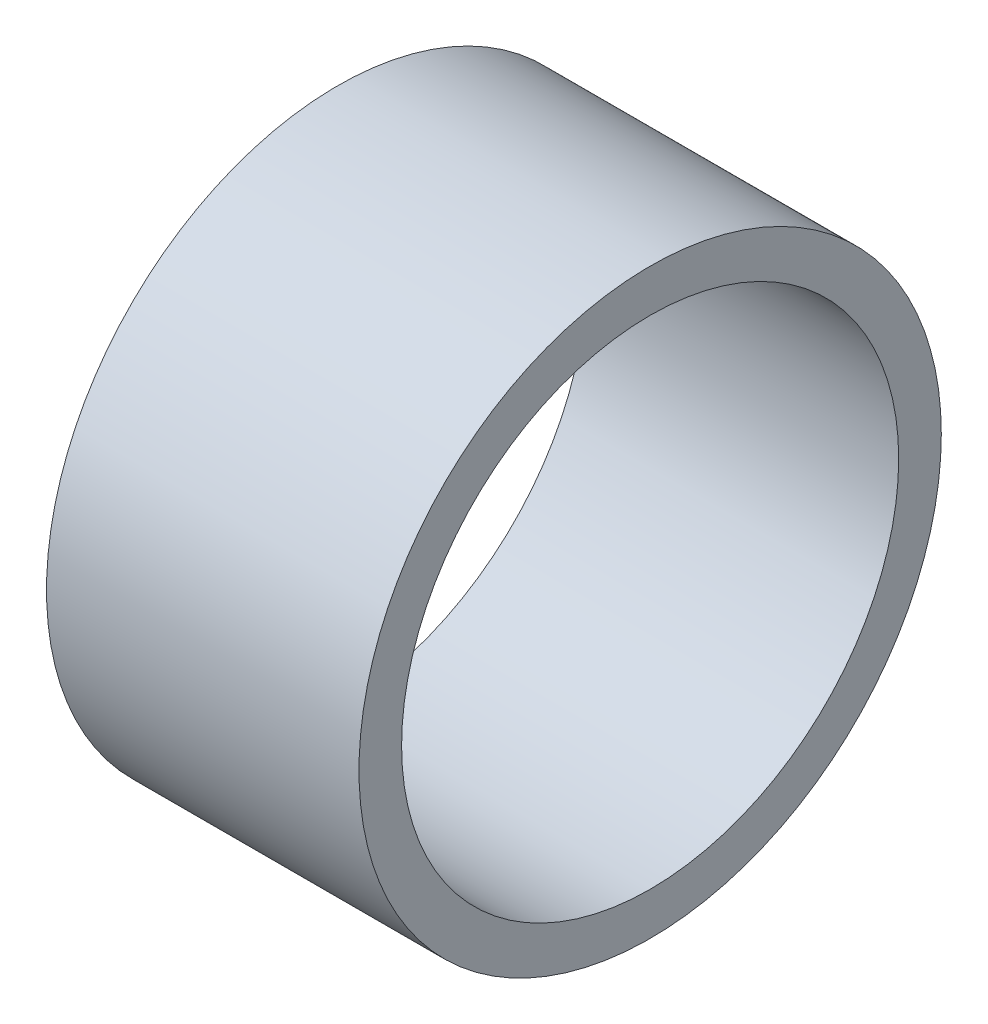
from build123d import *

# Parameters (mm, degrees)
SKETCH_1_R      = 20.5
SKETCH_1_R_2    = 17.5
EXTRUDE_1_DEPTH = 22


with BuildPart() as part:
    # 草图1 → 凸台-拉伸1 (new body)
    with BuildSketch(Plane(origin=(0, 0, 0), x_dir=(0, 0, -1), z_dir=(1, 0, 0))):
        Circle(SKETCH_1_R)
        Circle(SKETCH_1_R_2, mode=Mode.SUBTRACT)
    extrude(amount=EXTRUDE_1_DEPTH)


solid = part.part
